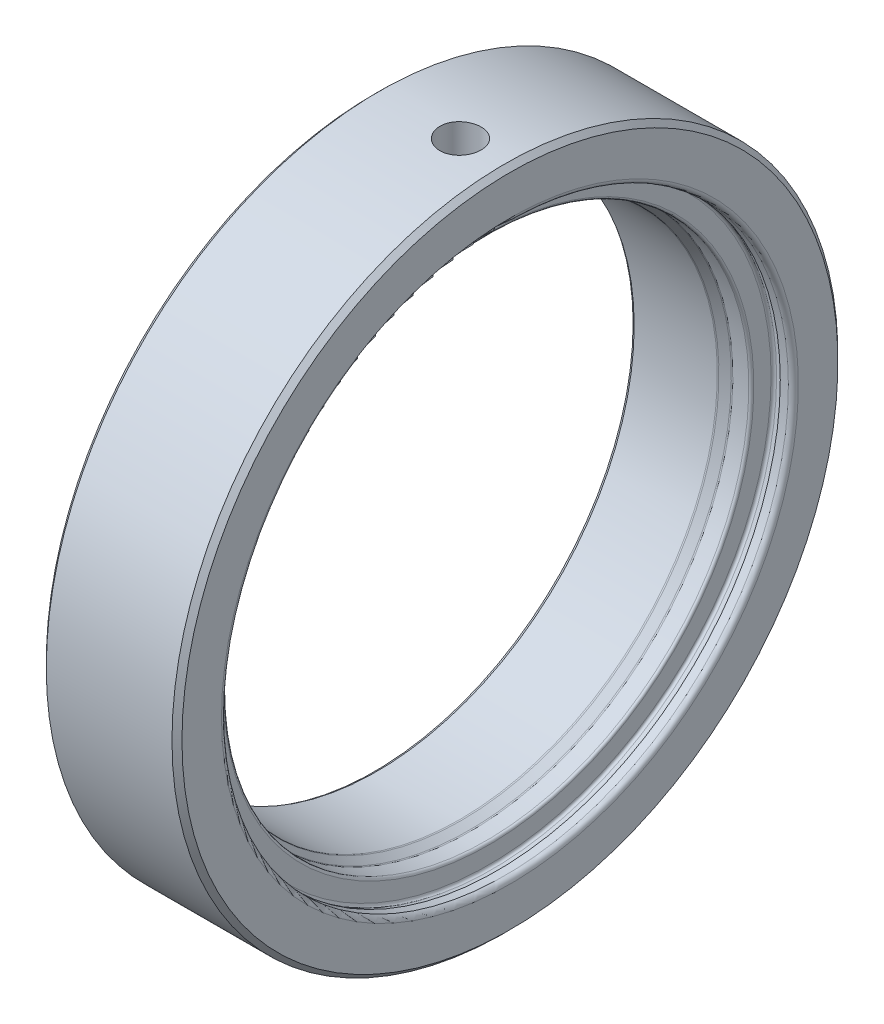
from build123d import *

# Parameters (mm, degrees)
CHAMFER2_SIZE                      = 0.762
CHAMFER2_SIZE2                     = 0.439940905
CHAMFER3_SIZE                      = 1.524
F_1_8_NPT_TAPPED_HOLE1_D           = 8.4328
F_1_8_NPT_TAPPED_HOLE1_DEPTH       = 63.119
F_1_8_NPT_TAPPED_HOLE1_CBORE_D     = 12.5731524
F_1_8_NPT_TAPPED_HOLE1_CBORE_DEPTH = 58.42
F_1_8_NPT_TAPPED_HOLE1_TIP         = 2.533468714


with BuildPart() as part:
    # Sketch1 → Revolve1 (revolve)
    with BuildSketch(Plane.XY, mode=Mode.PRIVATE) as revolve1_sk:
        with BuildLine():
            Line((0, 101.6), (41.402, 101.6))
            Line((41.402, 101.6), (41.402, 88.011))
            ThreePointArc((41.402, 88.011), (40.955630735, 86.933369265), (39.878, 86.487))
            Line((39.878, 86.487), (37.400925561, 86.487))
            Line((37.400925561, 86.487), (35.884220112, 86.8934))
            ThreePointArc((35.884220112, 86.8934), (35.223123791, 86.761899766), (34.925, 86.15736452))
            Line((34.925, 86.15736452), (34.925, 80.899))
            ThreePointArc((34.925, 80.899), (34.701815367, 80.360184633), (34.163, 80.137))
            Line((34.163, 80.137), (29.293607942, 80.137))
            ThreePointArc((29.293607942, 80.137), (29.096387829, 80.11103548), (28.912607942, 80.034911358))
            Line((28.912607942, 80.034911358), (26.516622715, 78.651588642))
            ThreePointArc((26.516622715, 78.651588642), (26.332842828, 78.57546452), (26.135622715, 78.5495))
            Line((26.135622715, 78.5495), (0, 78.5495))
            Line((0, 78.5495), (0, 101.6))
        make_face()
    revolve(revolve1_sk.sketch.rotate(Axis((-48.080119454, 0, 0), (1, 0, 0)), 90), axis=Axis((-48.080119454, 0, 0), (1, 0, 0)))

    # Chamfer2
    chamfer2_edges = [part.edges().sort_by_distance(p)[0] for p in [
        (0, 0, -78.5495),
    ]]
    chamfer2_side = [part.faces().sort_by_distance(p)[0] for p in [
        (13.067811358, 0, -78.5495),
    ]]
    chamfer(chamfer2_edges, length=CHAMFER2_SIZE, length2=CHAMFER2_SIZE2, reference=chamfer2_side[0])

    # Chamfer3
    chamfer3_edges = [part.edges().sort_by_distance(p)[0] for p in [
        (41.402, 0, -101.6),
        (0, 0, -101.6),
    ]]
    chamfer(chamfer3_edges, length=CHAMFER3_SIZE)

    # 1/8 NPT Tapped Hole1
    with Locations(Plane(origin=(26.3144, 101.6, 0), x_dir=(0, 0, 1), z_dir=(0, 1, 0))):
        with Locations((0, 0)):
            CounterBoreHole(F_1_8_NPT_TAPPED_HOLE1_D / 2, F_1_8_NPT_TAPPED_HOLE1_CBORE_D / 2, F_1_8_NPT_TAPPED_HOLE1_CBORE_DEPTH, depth=F_1_8_NPT_TAPPED_HOLE1_DEPTH)
            with Locations((0, 0, -(F_1_8_NPT_TAPPED_HOLE1_DEPTH + F_1_8_NPT_TAPPED_HOLE1_TIP / 2))):  # 118° drill point
                Cone(0, F_1_8_NPT_TAPPED_HOLE1_D / 2, F_1_8_NPT_TAPPED_HOLE1_TIP, mode=Mode.SUBTRACT)


solid = part.part
